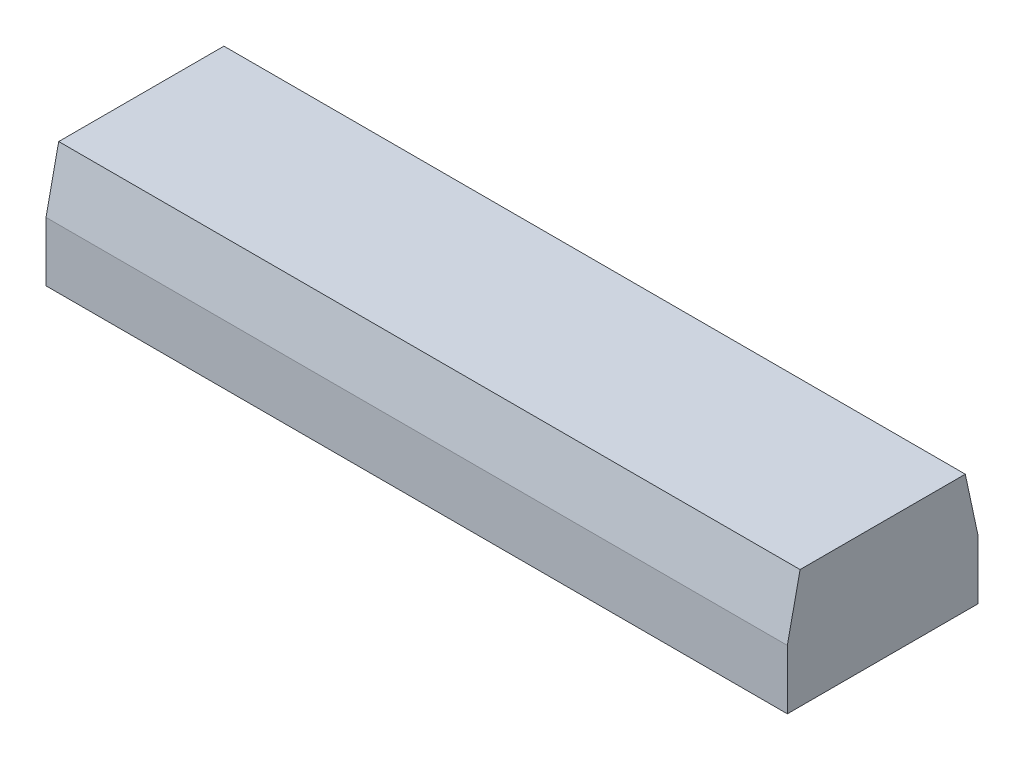
SolidWorks part; units mm, degrees
ref_plane "Front Plane" through (0, 0, 0) normal (0, 0, 1) x (1, 0, 0)
ref_plane "Top Plane" through (0, 0, 0) normal (0, 1, 0) x (1, 0, 0)
ref_plane "Right Plane" through (0, 0, 0) normal (1, 0, 0) x (0, 0, -1)
sketch "Sketch1" plane through (0, 0, 0) normal (0, 0, 1) x (1, 0, 0)
  line L1 (0, 0) -> (175, 0)
  line L2 (0, 0) -> (0, -28)
  line L3 (0, -28) -> (175, -28)
  line L4 (175, 0) -> (175, -28)
  dimension "D1" = 28
  dimension "D2" = 175
extrude "Boss-Extrude1" add sketch "Sketch1" along normal blind 45
hole_wizard "M8 Tapped Hole1" positions "Sketch4" profile "Sketch5" tap size "M8" standard "GB"
sketch "Sketch4" plane through (0, -28, 0) normal (0, -1, 0) x (-1, 0, 0)
  line L3 (-87.5, 0) -> (-87.5, -13.1998) construction
  line L6 (0, 0) -> (-175, 0) construction
  line L7 (-175, 0) -> (0, 0) construction
  point P0 (-27.5, -21)
  point P2 (-147.5, -21)
  dimension "D1" = 120
  dimension "D2" = 21
sketch "Sketch5" plane through (27.5, -28, 21) normal (1, 0, 0) x (0, 0, -1)
  line L0 (0, 0) -> (0, 21.7929)
  line L1 (0, 21.7929) -> (3.4, 19.75)
  line L2 (3.4, 19.75) -> (3.4, 0)
  line L5 (3.4, 0) -> (0, 0)
  line L10 (0, 21.7929) -> (-3.4, 19.75) construction
  line L11 (0, -6.35) -> (0, 107.95) construction
  dimension "螺纹孔钻头直径" = 6.8
  dimension "螺纹孔钻头深度" = 19.75
  dimension "导头角度" = 118
sketch "Sketch7" plane through (0, 0, 0) normal (-1, 0, 0) x (0, 0, 1)
  line L0 (3, 0) -> (0, -14)
  line L1 (45, 0) -> (0, 0) construction
  line L2 (0, 0) -> (0, -28) construction
  line L3 (0, -14) -> (0, 0)
  line L4 (0, 0) -> (3, 0)
  line L5 (22.5, 0) -> (22.5, -2.6436) construction
  line L6 (45, 0) -> (42, 0)
  line L7 (45, -14) -> (45, 0)
  line L8 (42, 0) -> (45, -14)
  line L9 (45, -28) -> (0, -28) construction
  dimension "D1" = 39
  dimension "D2" = 14
extrude "Cut-Extrude1" cut sketch "Sketch7" against normal through all
